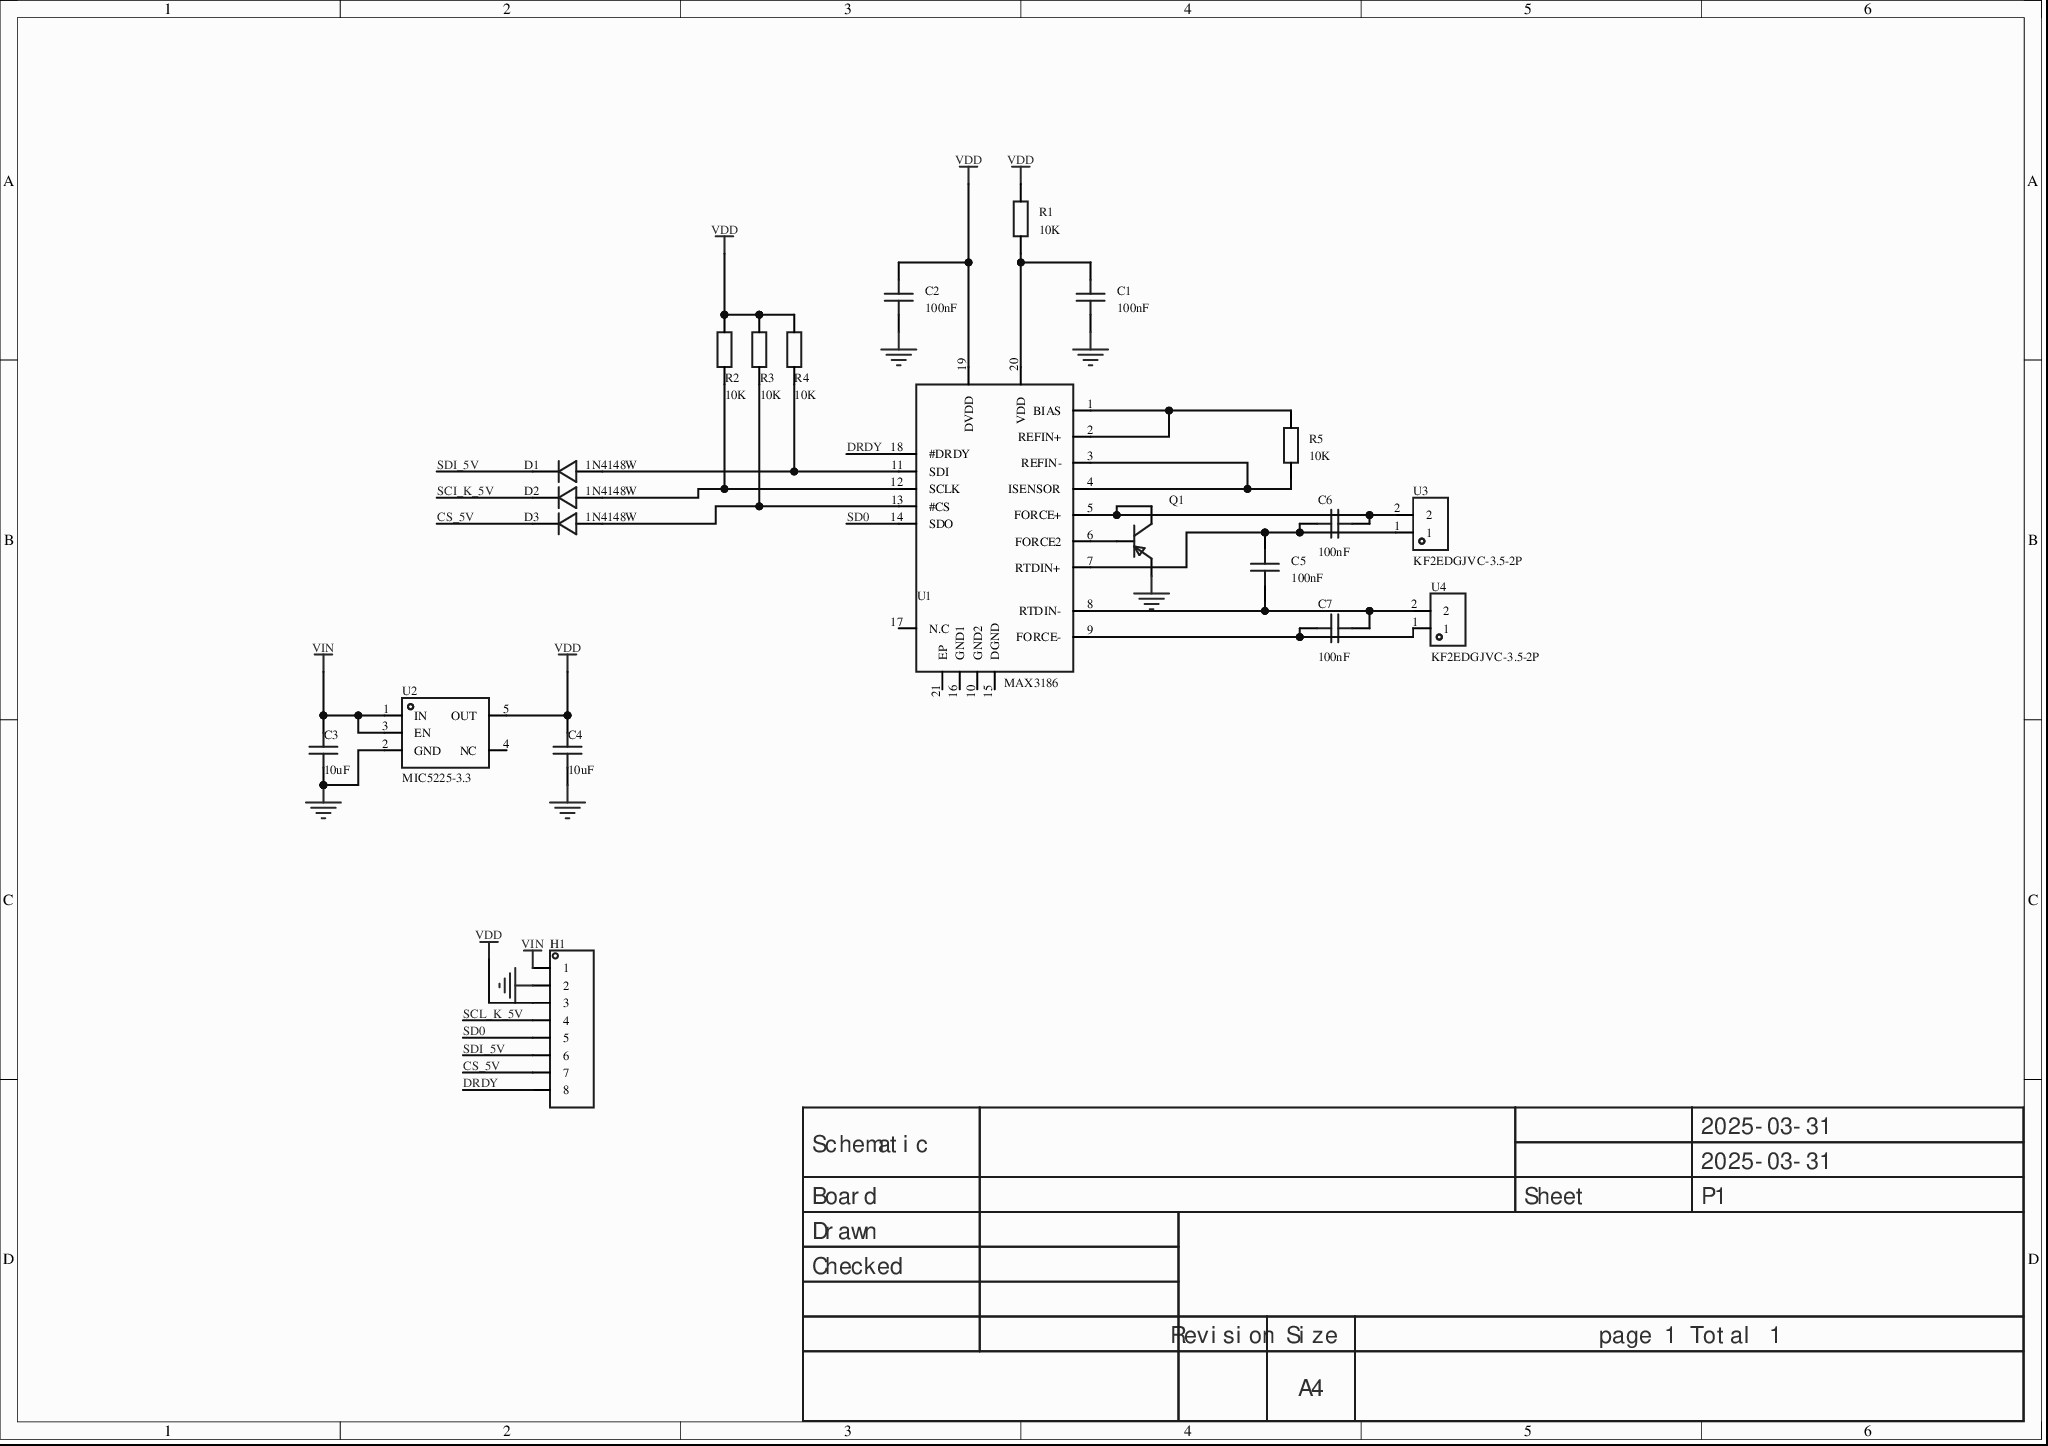
[diagram p0: MISC82906-3.schdoc]
# Altium project MISC82906-2.PrjPcb
1 sheet, 21 parts. Net scope: global (net labels, ports and power ports of the same name join across sheets).
Board file: MISC82906.pcbdoc

## Sheet MISC82906-3.schdoc
size 297 x 209 mm; Version: V1.0; @Project Name: MISC82906; @Page Count: 1; @Update Date: 2025-03-31; @Create Date: 2025-03-31; @Schematic Name: MISC82906; @Page No: 1; @Create Time: 12:48:31; @Update Time: 15:28:27; @Board Name: MISC82906

### Parts
C1  100nF  [C0603]
C2  100nF  [C0603]
C3  10uF  [C0603]
C4  10uF  [C0603]
C5  100nF  [C0603]
C6  100nF  [C0603]
C7  100nF  [C0603]
D1  1N4148W  [SOD-123F_L2.7-W1.6-LS3.8-RD]
D2  1N4148W  [SOD-123F_L2.7-W1.6-LS3.8-RD]
D3  1N4148W  [SOD-123F_L2.7-W1.6-LS3.8-RD]
H1  (no value)  [HDR-TH_8P-P2.54-V-M]
Q1  (no value)  [S8550P_SOT]
R1  10K  [R0603]
R2  10K  [R0603]
R3  10K  [R0603]
R4  10K  [R0603]
R5  10K  [R0603]
U1  MAX3186  [QFN-20_L5.0-W5.0-P0.65-BL-EP]
U2  MIC5225-3.3  [SOT-23-5_L3.0-W1.7-P0.95-LS2.8-BL]
U3  KF2EDGJVC-3.5-2P  [CONN-TH_2P-P3.50_KEFA_KF2EDGJVC-3.5-2P]
U4  KF2EDGJVC-3.5-2P  [CONN-TH_2P-P3.50_KEFA_KF2EDGJVC-3.5-2P]

### Nets
GND: C1.1 C2.1 C3.1 C4.1 H1.2 Q1.2(E) U2.2(GND)
VDD: C2.2 C4.2 H1.3 R1.2 R2.2 R3.2 R4.2 U1.19(DVDD) U2.5(OUT)
VIN: C3.2 H1.1 U2.1(IN) U2.3(EN)
CS_5V: D3.1(K) H1.7
DRDY: H1.8 U1.18(#DRDY)
SCI_K_5V: D2.1(K)
SCL_K_5V: H1.4
SD0: H1.5 U1.14(SDO)
SDI_5V: D1.1(K) H1.6
NetC1_2: C1.2 R1.1 U1.20(VDD)
NetC5_1: C5.1 C7.2 U1.8(RTDIN-) U4.2
NetC5_2: C5.2 C6.1 U1.7(RTDIN+) U3.1
NetC6_2: C6.2 Q1.3(C) U1.5(FORCE+) U3.2
NetC7_1: C7.1 U1.9(FORCE-) U4.1
NetD1_2: D1.2(A) R4.1 U1.11(SDI)
NetD2_2: D2.2(A) R2.1 U1.12(SCLK)
NetD3_2: D3.2(A) R3.1 U1.13(#CS)
NetQ1_1: Q1.1(B) U1.6(FORCE2)
NetR5_1: R5.1 U1.3(REFIN-) U1.4(ISENSOR)
NetR5_2: R5.2 U1.1(BIAS) U1.2(REFIN+)

Not connected (* = marked no-connect by the designer): U1 10(GND2) 15(DGND) 16(GND1) 17(N.C) 21(EP); U2 4(NC)*

### Notes on the sheet
- 2025-03-31
- Schematic
- Board
- Sheet
- P1
- Drawn
- Checked
- Revision
- Size
- A4
- page 1 Total 1

### Library data of the parts
C1-C7 = CAP_0603: ConvertToPcb: yes; SymbolName: CapAcitance; ModelId: ac125912035d415993ca9572d50418b1; ModelName: C0603_L1.6-W0.8-H0.8; ModelTransform: 62.992,31.496,0,0,0,0,0,0,0; Device: CAP_0603; AddInBom: yes; Supplier Footprint: 0603; FootprintName: C0603
  C1 C2 C5-C7: Value: 100nF
  C3 C4: Value: 10uF
D1-D3 = 1N4148W_C81598: Diode configuration: independent; forward voltage (Vf): 1V@50mA; DC reverse voltage (Vr): 75V; rectified current: 150mA; reverse recovery time (trr): 4ns;; Manufacturer: ST(先科); AddInBom: yes; ModelId: 7091c985327f41e7b1e4fbd3002f031e; ModelTransform: 149.606,62.992,0,0,0,0,0,0,0; Reverse Leakage Current (Ir): 1uA@75V; Symbol: 1N4148W_C81598; Device: 1N4148W_C81598; LCSC Part Name: 1N4148W; SupplierPart: C81598; ManufacturerPart: 1N4148W; Supplier Footprint: SOD-123; Datasheet: https://atta.szlcsc.com/upload/public/pdf/source/20161024/1477288446905.pdf; Supplier: LCSC; ConvertToPcb: yes; FootprintName: SOD-123F_L2.7-W1.6-LS3.8-RD; ModelName: SOD-123F_L2.7-W1.6-LS3.8-RD; Diode Configuration: Independent; Forward Voltage (Vf@If): 1V@50mA; Reverse Voltage (Vr): 75V; Rectified Current: 150mA; Reverse Recovery Time (trr): 4ns; Operating Temperature: -
H1 = HDR-M_2.54_1x8P: Symbol: Header-Male-2.54_1x8; ConvertToPcb: yes; ModelId: f5b96e27511e49e38545e53df2320202; ModelTransform: 807.87244,98.425,0,0,0,0,0,0,-118.11; Device: HDR-M_2.54_1x8P; AddInBom: yes; SupplierPart: C124381; Supplier Footprint: 插件; FootprintName: HDR-TH_8P-P2.54-V-M; ModelName: HDR-TH_8P-P2.54-V-M
Q1 = S8550_SOT_PNP: Symbol: PNP; ConvertToPcb: yes; ModelId: 9c0df02d6f3e44e889da37f3e5bf5496; ModelName: SOT-23-3_L2.9-W1.4-P1.90-LS2.5-BR; ModelTransform: 98.43,114.17,37.91,0,0,0,0,0,0; Device: S8550_SOT_PNP; AddInBom: yes; Supplier Footprint: SOT-23; FootprintName: S8550P_SOT
R1-R5 = Res_0603: ConvertToPcb: yes; SymbolName: Resistor; ModelId: fc143cca1e79419f9cd78b61e9279f08; ModelTransform: 31.8897,63.7794,0,90,0,0,0,0,0; Device: Res_0603; AddInBom: yes; Supplier Footprint: 0603; FootprintName: R0603; ModelName: R0603; Value: 10K
U1 = MAX31865ATP+T: Interface: SPI; supply voltage: 3V~3.6V; sampling rate: -; resolution: 15;; Manufacturer: ADI(亚德诺)/MAXIM(美信); AddInBom: yes; number of channels: 1; Integral nonlinearity: ±1LSB; resolution: 15; ModelId: f353a776191646bb88f03a12d834972c; ModelName: QFN-20_L5.0-W5.0-H1.0-P0.65; ModelTransform: 197.6374,197.6374,0,90,0,0,0.0005,0,0; Manufacturer Part: MAX3186; Symbol: MAX31865ATP+T; Device: MAX31865ATP+T; LCSC Part Name: MAX31865ATP; SupplierPart: C118474; Supplier Footprint: QFN-20-EP(5x5); JLCPCB Part Class: Extended library; Datasheet: https://atta.szlcsc.com/upload/public/pdf/source/20190723/C404011_F7F4B1E2DB54BAF2C7538ADE86C8BDC0.pdf; Supplier: LCSC; ConvertToPcb: yes; differential input: Yes; Supply Voltage: 3V~3.6V; sampling frequency: -; Operating Temperature: -40℃~+125℃; FootprintName: QFN-20_L5.0-W5.0-P0.65-BL-EP
U2 = MIC5225-3.3YM5-TR: Output type: fixed; max input voltage: 16V; output voltage: 3.3V; output current: 150mA; output polarity: positive;; Manufacturer: MICROCHIP(美国微芯); AddInBom: yes; Dropout Voltage: 450mV@(150mA); Number of Outputs: 1; ModelId: 0a2a1b8f50944f73965918ad6e5fe167; ModelName: SOT-23-5_L2.9-W1.6-H1.1-LS2.8-P0.95; ModelTransform: 118.60433,114.173,0,90,0,0,0.0005,0.0005,0; Manufacturer Part: MIC5225-3.3; Symbol: MIC5225-3.3YM5-TR; Device: MIC5225-3.3YM5-TR; LCSC Part Name: 超低静态电流150mA低压差稳压器; SupplierPart: C512101; Supplier Footprint: SOT-23-5; JLCPCB Part Class: Extended library; Datasheet: https://atta.szlcsc.com/upload/public/pdf/source/20200413/C512101_F5C0F3AED6CD09592E1975F2BB445A54.pdf; Supplier: LCSC; ConvertToPcb: yes; Output Type: Fixed; Maximum Input Voltage: 16V; Output Voltage: 3.3V; Output Current: 150mA; Feature: ESD protection; thermal shutdown (TSD); reverse polarity protection; overcurrent protection (OCP); enable; Operating Temperature: -40℃~+125℃; Output Polarity: Positive; FootprintName: SOT-23-5_L3.0-W1.7-P0.95-LS2.8-BL
U3 U4 = KF2EDGJVC-3.5-2P: AddInBom: yes; ModelId: 14fdc3c25ad14b70b67ca6c4678e6866; ModelTransform: 330.708,295.669,0,0,0,0,0,10.512,-137.795; Symbol: KF2EDGJVC-3.5-2P; Device: KF2EDGJVC-3.5-2P; LCSC Part Name: KF2EDGJVC-3.5-2P; SupplierPart: C9900094985; ManufacturerPart: KF2EDGJVC-3.5-2P; Supplier Footprint: CONN-TH_3P-P3.50_KEFA_KF2EDGJVC-3.5-2P; JLCPCB Part Class: Extended library; Supplier: LCSC; ConvertToPcb: yes; FootprintName: CONN-TH_2P-P3.50_KEFA_KF2EDGJVC-3.5-2P; ModelName: CONN-TH_2P-P3.50_KEFA_KF2EDGJVC-3.5-2P